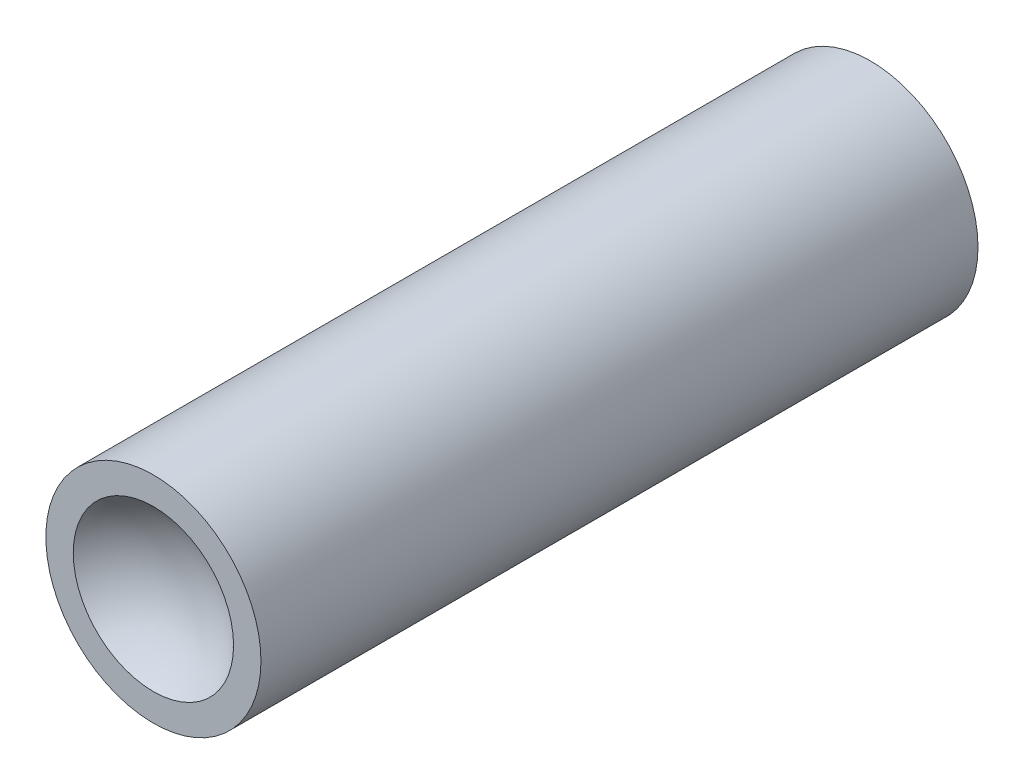
from build123d import *

# Parameters (mm, degrees)
SKETCH_1_R      = 6
EXTRUDE_1_DEPTH = 40


with BuildPart() as part:
    # 草图1 → 凸台-拉伸1 (new body)
    with BuildSketch(Plane.XY):
        Circle(SKETCH_1_R)
    extrude(amount=EXTRUDE_1_DEPTH)

    # 草图2 → 切除-旋转4 (revolve, cut)
    with BuildSketch(Plane(origin=(0, 0, 0), x_dir=(1, 0, 0), z_dir=(0, 1, 0))):
        with BuildLine():
            Line((0, -50), (0, -38))
            ThreePointArc((0, -38), (-6, -44), (0, -50))
        make_face()
    revolve(axis=Axis((0, 0, 50), (0, 0, -1)), mode=Mode.SUBTRACT)


solid = part.part
